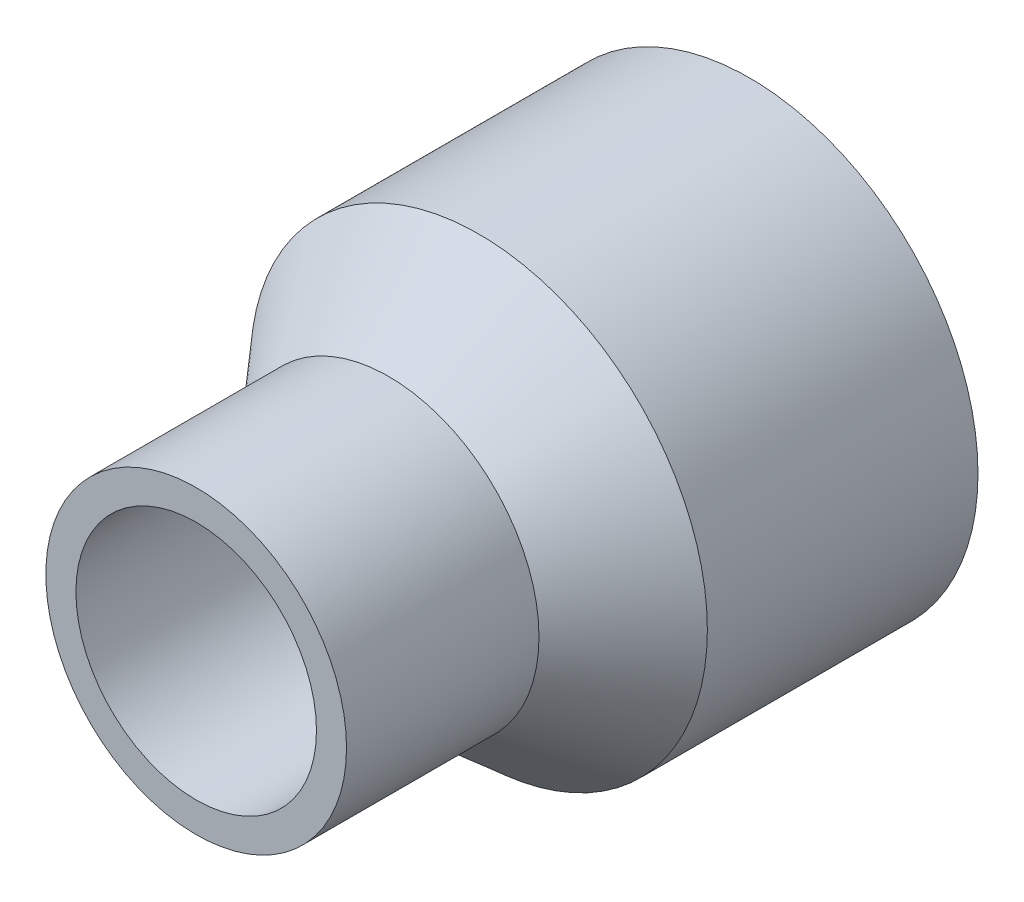
SolidWorks part; units mm, degrees
material "PP 共聚物"
ref_plane "前视基准面" through (0, 0, 0) normal (0, 0, 1) x (1, 0, 0)
ref_plane "上视基准面" through (0, 0, 0) normal (0, 1, 0) x (1, 0, 0)
ref_plane "右视基准面" through (0, 0, 0) normal (1, 0, 0) x (0, 0, -1)
sketch "草图1" plane through (0, 0, 0) normal (1, 0, 0) x (0, 0, -1)
  line L0 (0, 0) -> (139.2221, 0) construction
  line L1 (53.6111, 10) -> (69.6111, 10)
  line L2 (69.6111, 10) -> (77.1111, 16)
  line L3 (77.1111, 16) -> (99.6111, 16)
  line L4 (53.6111, 10) -> (53.6111, 12.5)
  line L5 (53.6111, 12.5) -> (69.6111, 12.5)
  line L6 (69.6111, 12.5) -> (77.1111, 19)
  line L7 (77.1111, 19) -> (99.6111, 19)
  line L9 (99.6111, 16) -> (99.6111, 19)
  dimension "D1" = 10
  dimension "D2" = 16
  dimension "D3" = 16
  dimension "D4" = 22.5
  dimension "D5" = 46
  dimension "D6" = 12.5
  dimension "D7" = 19
revolve "旋转1" add sketch "草图1" angle 360 about L0
